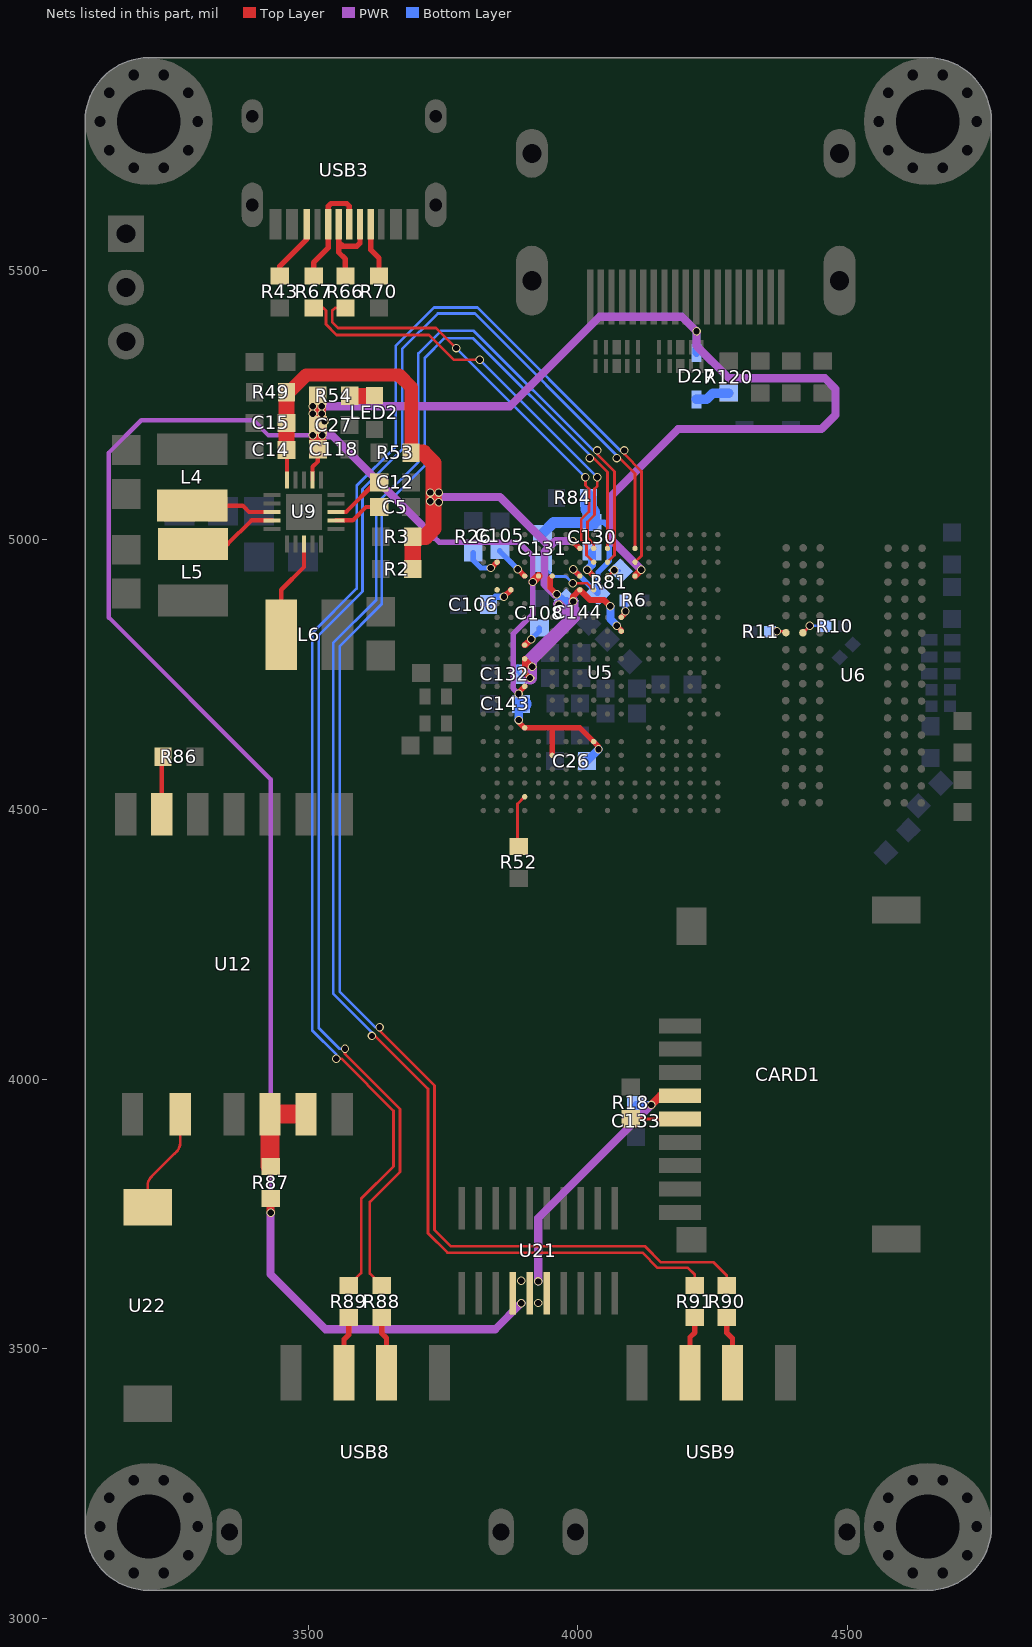
[diagram p0: the nets of this part, all layers, seen from the top]
# Altium PCB MISC105417.pcbdoc (part 2 of 5)
Units mil, origin at the board's own origin, x right, y up, seen from the top; angles counter-clockwise.
Board outline 1681.1 x 2842.52 mil, 4 copper layers (Top Layer, GND, PWR, Bottom Layer), stack 62.447 mil thick; 102 components, 152 nets, 737 pads, 611 vias.

## Footprints (in the part's own frame and the unit in brackets; to place one, negate y for a bottom-side part, rotate by r counter-clockwise, add the part's x,y. Pads: shape width x height; smd on the part's side, far side on the other; paste and mask are expansions set on the pad) (continued)
FBGA96 [mil]
  round 14 smd: A1(-128.47,241.36) A2(-96.97,241.37) A3(-65.47,241.38) A7(60.53,241.42) A8(92.03,241.43) A9(123.53,241.44) B1(-128.46,209.86) B2(-96.96,209.87) B3(-65.46,209.88) B7(60.54,209.92) B8(92.04,209.93) B9(123.54,209.94) C1(-128.46,178.36) C2(-96.96,178.37) C3(-65.46,178.38) C7(60.54,178.42) C8(92.04,178.43) C9(123.54,178.44) D1(-128.45,146.86) D2(-96.95,146.87) D3(-65.45,146.88) D7(60.55,146.92) D8(92.05,146.93) D9(123.55,146.94) E1(-128.44,115.36) E2(-96.94,115.37) E3(-65.44,115.38) E7(60.56,115.42) E8(92.06,115.43) E9(123.56,115.44) F1(-128.43,83.86) F2(-96.93,83.87) F3(-65.43,83.88) F7(60.57,83.92) F8(92.07,83.93) F9(123.57,83.94) G1(-128.42,52.36) G2(-96.92,52.37) G3(-65.42,52.38) G7(60.58,52.42) G8(92.08,52.43) G9(123.58,52.44) H1(-128.41,20.86) H2(-96.91,20.87) H3(-65.41,20.88) H7(60.59,20.92) H8(92.09,20.93) H9(123.59,20.94) J1(-128.4,-10.64) J2(-96.9,-10.63) J3(-65.4,-10.62) J7(60.6,-10.58) J8(92.1,-10.57) J9(123.6,-10.56) K1(-128.39,-42.14) K2(-96.89,-42.13) K3(-65.39,-42.12) K7(60.61,-42.08) K8(92.11,-42.07) K9(123.61,-42.06) L1(-128.38,-73.64) L2(-96.88,-73.63) L3(-65.38,-73.62) L7(60.62,-73.58) L8(92.12,-73.57) L9(123.62,-73.56) M1(-128.37,-105.14) M2(-96.87,-105.13) M3(-65.37,-105.12) M7(60.63,-105.08) M8(92.13,-105.07) M9(123.63,-105.06) N1(-128.36,-136.64) N2(-96.86,-136.63) N3(-65.36,-136.62) N7(60.64,-136.58) N8(92.14,-136.57) N9(123.64,-136.56) P1(-128.35,-168.14) P2(-96.85,-168.13) P3(-65.35,-168.12) P7(60.65,-168.08) P8(92.15,-168.07) P9(123.65,-168.06) R1(-128.34,-199.64) R2(-96.84,-199.63) R3(-65.34,-199.62) R7(60.66,-199.58) R8(92.16,-199.57) R9(123.66,-199.56) T1(-128.33,-231.14) T2(-96.83,-231.13) T3(-65.33,-231.12) T7(60.67,-231.08) T8(92.17,-231.07) T9(123.67,-231.06)
  silkscreen extent -180,-270 175,281
HDMI-SMD_HDMI-19PIN-043 [mm]
  rect 0.3x2.6 smd paste-100 mask+0.05: 1(4.5,3.38) 2(4,3.38) 3(3.5,3.38) 4(3,3.38) 5(2.5,3.38) 6(2,3.38) 7(1.5,3.38) 8(1,3.38) 9(0.5,3.38) 10(0,3.38) 11(-0.5,3.38) 12(-1,3.38) 13(-1.5,3.38) 14(-2,3.38) 15(-2.5,3.38) 16(-3,3.38) 17(-3.5,3.38) 18(-4,3.38) 19(-4.5,3.38)
  oval 1.5x2.3 hole 0.9 slot 1.7 at 90 deg paste+0 mask+0.05: 20(-7.25,-3.38) 20(7.25,-3.38)
  oval 1.5x3.3 hole 0.9 slot 2.7 at 90 deg paste+0 mask+0.05: 20(-7.25,2.62) 20(7.25,2.62)
  silkscreen extent -7.5,-7.88 7.5,4.92
hdr-th_3p-p2.54-v-m [mm]
  rect 1.7x1.7 hole 0.889 paste+0 mask+0.051: 1(-2.54,0)
  round 1.7 hole 0.889 paste+0 mask+0.051: 2(0,0) 3(2.54,0)
  silkscreen extent -4.02,-1.27 4.02,1.27
IND-SMD_L3.0-W3.0 [mm]
  rect 1.5x3.32 smd paste+0 mask+0.051: 1(1.328,0) 2(-1.328,0)
  silkscreen extent -1.52,-1.91 1.52,1.91
LED_0603 [mil]
  rect 31.5x31.5 smd paste+0 mask+2: 1(-33.5,-0.4) 2(29.5,-0.2)
  silkscreen extent -61,-30 53,30
M3_HOLE [mm]
  round 1 hole 0.5: 1(-2.3,0) 1(-1.861,-1.352) 1(-1.861,1.352) 1(-0.711,-2.187) 1(-0.711,2.187) 1(0.711,-2.187) 1(0.711,2.187) 1(1.861,-1.352) 1(1.861,1.352) 1(2.3,0)
  round 6 hole 3: 1(0,0)
OSC-SMD_4P-L2.0-W1.6-BL [mil]
  rect 30x20 smd: 1(-25,-20) 2(25,-20) 3(25,20) 4(-25,20)
R0402 [mm]
  rect 0.566x0.54 smd paste-100 mask+0.051: 1(-0.433,0) 2(0.433,0)
  silkscreen extent -0.94,-0.5 0.94,0.5
R0402-NSK_2 [mil]
  rect 19.68x22 smd paste+0 mask+2: 1(-18,0) 2(18,0)
R0603 [mil]
  rect 31.75x34.02 smd paste-3937.01 mask+2: 1(-29.66,0) 2(29.66,0)
  silkscreen extent -55,-26 55,26
SLP2510P8_L2.5-W1.0-P0.50-BL [mil]
  rect 7.9x26.8 smd paste+0 mask+2: 1(-39.4,-17.3) 2(-19.7,-17.3) 4(19.7,-17.3) 5(39.4,-17.3) 6(39.4,17.3) 7(19.7,17.3) 9(-19.7,17.3) 10(-39.4,17.3)
  rect 15.7x26.8 smd paste+0 mask+2: 3(0,-17.3) 8(0,17.3)
  silkscreen extent -57,-35 51,22
SOD-323_L1.8-W1.3-LS2.5-NSK [mil]
  rect 33.3x17.9 smd paste+0 mask+2: 1(-43.2,0) 2(43.2,0)
  silkscreen extent -18,-10 -6,7
TF-SMD_TF-015 [mil]
  rect 27.6x78.7 smd paste+0 mask+2: 1(90.7,200.6) 2(47.6,200.5) 3(4.4,200.6) 4(-38.8,200.6) 5(-82.1,200.6) 6(-125.3,200.6) 7(-168.5,200.6) 8(-211.7,200.6) 9(-255.2,200.6)
  rect 47.2x55 smd paste+0 mask+2: 10(-305.7,179.4)
  rect 50x90 smd paste+0 mask+2: 11(-304.3,-200.6) 12(305.7,-200.6)
  rect 70x55 smd paste+0 mask+2: 13(275.7,179.4)
  Board Outline Layer circle w0.1: c-192.8,-216.8 r19.7
  Board Outline Layer circle w0.1: c122.1,-216.7 r19.7
  Board Outline Layer region: -192.8,-236.5 -201.35,-234.55 -208.2,-229.08 -212.01,-221.18 -212.01,-212.42 -208.2,-204.52 -201.35,-199.05 -192.8,-197.1 -192.8,-197.1 -184.25,-199.05 -177.4,-204.52 -173.59,-212.42 -173.59,-221.18 -177.4,-229.08 -184.25,-234.55 -192.8,-236.5
  Board Outline Layer region: -192.8,-236.5 -196.64,-236.12 -200.34,-235 -203.74,-233.18 -206.73,-230.73 -209.18,-227.74 -211,-224.34 -212.12,-220.64 -212.5,-216.8 -212.12,-212.96 -211,-209.26 -209.18,-205.86 -206.73,-202.87 -203.74,-200.42 -200.34,-198.6 -196.64,-197.48 -192.8,-197.1 -188.96,-197.48 -185.26,-198.6 -181.86,-200.42 -178.87,-202.87 -176.42,-205.86 -174.6,-209.26 -173.48,-212.96 -173.1,-216.8 -173.48,-220.64 -174.6,-224.34 -176.42,-227.74 -178.87,-230.73 -181.86,-233.18 -185.26,-235 -188.96,-236.12
  Board Outline Layer region: 122.1,-236.4 113.55,-234.45 106.7,-228.98 102.89,-221.08 102.89,-212.32 106.7,-204.42 113.55,-198.95 122.1,-197 122.1,-197 130.65,-198.95 137.5,-204.42 141.31,-212.32 141.31,-221.08 137.5,-228.98 130.65,-234.45 122.1,-236.4
  Board Outline Layer region: 122.1,-236.4 118.26,-236.02 114.56,-234.9 111.16,-233.08 108.17,-230.63 105.72,-227.64 103.9,-224.24 102.78,-220.54 102.4,-216.7 102.78,-212.86 103.9,-209.16 105.72,-205.76 108.17,-202.77 111.16,-200.32 114.56,-198.5 118.26,-197.38 122.1,-197 125.94,-197.38 129.64,-198.5 133.04,-200.32 136.03,-202.77 138.48,-205.76 140.3,-209.16 141.42,-212.86 141.8,-216.7 141.42,-220.54 140.3,-224.24 138.48,-227.64 136.03,-230.63 133.04,-233.08 129.64,-234.9 125.94,-236.02
  Multi-Layer board cut-out: -192.8,-236.5 -201.35,-234.55 -208.2,-229.08 -212.01,-221.18 -212.01,-212.42 -208.2,-204.52 -201.35,-199.05 -192.8,-197.1 -192.8,-197.1 -184.25,-199.05 -177.4,-204.52 -173.59,-212.42 -173.59,-221.18 -177.4,-229.08 -184.25,-234.55 -192.8,-236.5
  Multi-Layer board cut-out: 122.1,-236.4 113.55,-234.45 106.7,-228.98 102.89,-221.08 102.89,-212.32 106.7,-204.42 113.55,-198.95 122.1,-197 122.1,-197 130.65,-198.95 137.5,-204.42 141.31,-212.32 141.31,-221.08 137.5,-228.98 130.65,-234.45 122.1,-236.4
  silkscreen extent -287,-376 295,165
USB-A-SMD_C42496 [mm]
  rect 1x2.6 smd paste-100 mask+0.05: 1(-3.5,3.75) 2(-1,3.75) 3(1,3.75) 4(3.5,3.75)
  oval 1.2x2.2 hole 0.8 slot 1.8 at 90 deg paste+0 mask+0.05: 5(-6.4,-3.75) 6(6.4,-3.75)
  silkscreen extent -7.15,-6.25 7.15,3.75
USB-C-SMD_TYPEC-304-BCP16-1 [mil]
  oval 39.4x82.7 hole 23.6 slot 66.9 at 90 deg paste+0 mask+1.97: 12(-170.1,64.3) 13(170.1,64.3)
  oval 39.4x63 hole 23.6 slot 47.2 at 90 deg paste+0 mask+1.97: 14(-170.1,-100.3) 15(170.1,-100.3)
  rect 21.7x57.1 smd paste-3937.01 mask+1.97: A1B12(-127,100.3) A4B9(-96.5,100.3) B1A12(127,100.3) B4A9(96.5,100.3)
  rect 11.8x57.1 smd paste-3937.01 mask+1.97: A5(-49.2,100.3) A6(-9.8,100.3) A7(9.8,100.3) A8(49.2,100.3) B5(68.9,100.3) B6(29.5,100.3) B7(-29.5,100.3) B8(-68.9,100.3)
  Board Outline Layer circle w0.1: c-113.8,43.4 r12.8
  Board Outline Layer circle w0.1: c113.8,43.4 r12.8
  Board Outline Layer region: -126.6,43.4 -125.33,48.95 -121.78,53.41 -116.65,55.88 -110.95,55.88 -105.82,53.41 -102.27,48.95 -101,43.4 -101,43.4 -102.27,37.85 -105.82,33.39 -110.95,30.92 -116.65,30.92 -121.78,33.39 -125.33,37.85 -126.6,43.4
  Board Outline Layer region: -126.6,43.4 -126.23,46.46 -125.13,49.35 -123.38,51.89 -121.07,53.93 -118.34,55.37 -115.34,56.11 -112.26,56.11 -109.26,55.37 -106.53,53.93 -104.22,51.89 -102.47,49.35 -101.37,46.46 -101,43.4 -101.37,40.34 -102.47,37.45 -104.22,34.91 -106.53,32.87 -109.26,31.43 -112.26,30.69 -115.34,30.69 -118.34,31.43 -121.07,32.87 -123.38,34.91 -125.13,37.45 -126.23,40.34
  Board Outline Layer region: 101,43.4 102.27,48.95 105.82,53.41 110.95,55.88 116.65,55.88 121.78,53.41 125.33,48.95 126.6,43.4 126.6,43.4 125.33,37.85 121.78,33.39 116.65,30.92 110.95,30.92 105.82,33.39 102.27,37.85 101,43.4
  Board Outline Layer region: 101,43.4 101.37,46.46 102.47,49.35 104.22,51.89 106.53,53.93 109.26,55.37 112.26,56.11 115.34,56.11 118.34,55.37 121.07,53.93 123.38,51.89 125.13,49.35 126.23,46.46 126.6,43.4 126.23,40.34 125.13,37.45 123.38,34.91 121.07,32.87 118.34,31.43 115.34,30.69 112.26,30.69 109.26,31.43 106.53,32.87 104.22,34.91 102.47,37.45 101.37,40.34
  Multi-Layer board cut-out: -126.6,43.4 -125.33,48.95 -121.78,53.41 -116.65,55.88 -110.95,55.88 -105.82,53.41 -102.27,48.95 -101,43.4 -101,43.4 -102.27,37.85 -105.82,33.39 -110.95,30.92 -116.65,30.92 -121.78,33.39 -125.33,37.85 -126.6,43.4
  Multi-Layer board cut-out: 101,43.4 102.27,48.95 105.82,53.41 110.95,55.88 116.65,55.88 121.78,53.41 125.33,48.95 126.6,43.4 126.6,43.4 125.33,37.85 121.78,33.39 116.65,30.92 110.95,30.92 105.82,33.39 102.27,37.85 101,43.4
  silkscreen extent -173,-203 173,16
WIFI模块 [mm]
  rect 2x1 smd: 1(1.947,-1.15) 2(1.947,-2.85) 3(1.947,-4.55) 4(1.947,-6.25) 5(1.947,-7.95) 6(1.947,-9.65) 7(1.947,-11.35) 8(16.08,-11.03) 9(16.08,-8.78) 10(16.08,-6.25) 11(16.08,-4.55) 12(16.08,-2.85) 13(16.08,-1.15)
  silkscreen extent -0.3,-12.5 16.08,0
WQFN-20_L3.0-W3.0-P0.40-BL-EP [mil]
  rect 7.9x31.5 smd paste+0 mask+2: 1(-31.5,-59.1) 2(-15.8,-59.1) 3(0,-59.1) 4(15.7,-59.1) 5(31.5,-59.1) 11(31.5,59.1) 12(15.7,59.1) 13(0,59.1) 14(-15.8,59.1) 15(-31.5,59.1)
  rect 31.5x7.9 smd paste+0 mask+2: 6(59.1,-31.5) 7(59.1,-15.7) 8(59.1,0) 9(59.1,15.7) 10(59.1,31.5) 16(-59.1,31.5) 17(-59.1,15.8) 18(-59.1,0) 19(-59.1,-15.7) 20(-59.1,-31.5)
  rect 66.9x66.9 smd paste+0 mask+2: 21(0,0)
  silkscreen extent -61,-83 61,61

## Via types
v1: diameter 15.7, hole 11.8, Top Layer to Bottom Layer, 611 vias

## Nets (pads, with @x,y where several pads share a name; then routed paths per layer and width w, separated by ;. In a path a pad name is that pad's centre, name@x,y a point inside that pad or via, vN(x,y) a via of type N, cw(c..) or ccw(c..) an arc to the next point about the centre after c; other vN are vias at no path point)
1V8: C14.2 C15.2 C132.1 C144.2 R2.1 R3.1 R49.2 R53.1 U5.D11 U5.D12 U5.F18 U5.H17 U5.H20 U5.L14 U9.15 | length 1780.8
  Top Layer w8: C14.2@3459.53,5167 3460.5,5166.03 U9.15@3460.5,5111.1
  Top Layer w10: v1(3911.2,4743.94) 3911.2,4744.05 U5.D11@3901.25,4754 U5.D12@3901.25,4779.59 3915.2,4765.64 v1(3915.2,4764.94) ; U5.F18@3952.43,4933.13 3949,4929.7 3949,4910.97 v1(3960.65,4899.32) ; v1@3990,4997.92 U5.H20@4003.61,4984.31 ; v1(4072.2,4840.94) 4080.39,4832.77 U5.L14@4080.39,4830.77
  Top Layer w11: v1(3991.2,4885.94) 3991.2,4895.13 U5.H17@4003.61,4907.54 4022.21,4888.94 4048.2,4888.94 v1(4060.2,4876.94)
  Top Layer w25: R49.2@3459.66,5274 3464,5274 3496,5306 3668,5306 3690.66,5283.34 R53.1@3690.66,5162
  Top Layer w30: C14.2@3459.53,5167 3459.66,5167.13 R49.2@3459.66,5274 ; R53.1@3690.66,5162 3713,5162 3732,5143 3732,5021 3717,5006 R3.1@3693.66,5006 R2.1@3693.66,4946
  PWR w15: 3728,5080 3855.15,5080 3947.6,4987.54 ; v1(3960.65,4899.32) 3956.68,4899.32 3938,4918 3938,4977.94 3947.6,4987.54 ; v1(3990,4998) 3958.06,4998 3947.6,4987.54
  PWR w20: v1(3964.2,4879.94) 3975.83,4868.32 3991.2,4868.32 v1(3991.2,4885.94)
  PWR w25: v1(3911.2,4743.94) 3911.2,4776.94 3991.2,4856.94 3991.2,4868.32
  Bottom Layer w5: C132.1@3888.2,4766.94 3888.2,4754.79 C132.1@3892.08,4750.91 3892.08,4744.82 C132.1@3889.2,4741.94 ; C144.2@3978.64,4886.79 3979.49,4885.94 v1(3991.2,4885.94)
  Bottom Layer w10: v1(3964.2,4879.94) 3971.79,4879.94 C144.2@3978.64,4886.79
  Bottom Layer w15: v1(3960.65,4899.32) 3973.18,4886.79 C144.2@3978.64,4886.79 ; v1(4060.2,4876.94) 4060.2,4852.94 v1(4072.2,4840.94)
  other v1: 3742,5070 3726,5072 3726,5088 3742,5088
3V3: C26.2 C27.2 C118.2 C133.2 C143.2 CARD1.4 D27.2 R54.2 R87.1 U5.D7 U5.D10 U5.E18 U5.F5 U5.J6 U5.M18 U9.12 U21.4 U21.5 U21.6 | length 6238
  Top Layer w8: U9.12@3507.7,5111.1 3507.7,5135.7 3517.63,5145.63 C118.2@3517.63,5168.29
  Top Layer w10: v1(3889.91,4714.61) 3889.91,4717.07 U5.D10@3901.25,4728.41 ; v1(3890.2,4665.94) 3890.2,4662.69 U5.D7@3901.25,4651.64 3952.43,4651.64 ; U5.F5@3952.43,4600.46 3952.43,4651.64 ; v1(4038.2,4611.94) 4038.2,4617.05 U5.J6@4029.2,4626.05 4003.61,4651.64 3952.43,4651.64
  Top Layer w12: U5.M18@4105.98,4933.13 4117.2,4944.35 v1(4117.2,4944.94)
  Top Layer w15: v1(3430,3752) R87.1@3430,3778.34 ; v1(3916,4922) 3916,4922.29 U5.E18@3926.84,4933.13 ; v1(4136,3952) 4153.2,3969.2 CARD1.4@4189.4,3969.2
  Top Layer w30: R54.2@3517.5,5267.29 C27.2@3517.47,5213 3517.5,5168.42 C118.2@3517.63,5168.29
  PWR w8: v1(3430,3752) 3430,4556 3130,4856 3130,5162 3190,5222 3398.1,5222 3426.1,5194 v1(3508,5194)
  PWR w10: 3732.41,5006 3742.41,4996 3890,4996 3916,4970 v1(3916,4922) 3916,4862 3880,4826 3880,4724.52 v1(3889.91,4714.61)
  PWR w15: v1(3430,3752) 3430,3638 3532,3536 3846.63,3536 v1(3895,3584.37) ; v1(3508,5194) v1(3526.04,5194) 3544.41,5194 3732.41,5006 ; v1(3525.18,5248) 3874,5248 4040,5414 4193.19,5414 v1(4220,5387.19) 4220,5360 4280,5300 4458,5300 4478,5280 4478,5232 4452,5206 4186,5206 4063,5083 4063,4999.15 v1(4117.2,4944.94) ; v1(3926.44,3624.66) 3926.44,3742.44 v1(4136,3952)
  Bottom Layer w5: v1(3889.91,4714.61) 3889.91,4700.35 C143.2@3894.35,4695.91
  Bottom Layer w15: v1(3890.2,4665.94) 3890.2,4691.76 C143.2@3894.35,4695.91 ; C26.2@4016.73,4589.94 4038.2,4611.41 v1(4038.2,4611.94) ; C133.2@4108,3951.53 4108.47,3952 v1(4136,3952) ; D27.2@4220,5347.2 v1(4220,5387.19)
  Bottom Layer w30: C143.2@3894.35,4695.91 C143.2@3899.24,4695.91
  other v1: 3926.44,3584.66 3895,3626 3530,5220 3508,5234 3524.57,5234 3508,5248
$1N1032: R6.1 U5.L15 | length 35.5
  Top Layer w10: U5.L15@4080.39,4856.36 4088.2,4864.17 v1(4088.2,4867.94)
  Bottom Layer w10: R6.1@4086.52,4887.91 4086.52,4869.62 v1(4088.2,4867.94)
$1N2048: R10.2 U6.L8 | length 47.8
  Top Layer w5: U6.L8@4417.34,4827.89 4430.2,4840.76 v1(4430.2,4840.94)
  Bottom Layer w5: v1(4430.2,4840.94) 4458.16,4840.94 R10.2@4459.16,4839.94
$1N2049: R11.2 U6.L9 | length 17.9
  Top Layer w5: v1(4369.2,4830.94) 4382.89,4830.94 U6.L9@4385.84,4827.99
$2N1493: LED2.2 R54.1 | length 45.7
  Top Layer w30: R54.1@3576.82,5267.29 3621.86,5267.29 LED2.2@3622.36,5267.79
$2N1502: C12.2 U9.8 | length 103.2
  Top Layer w8: U9.8@3551.1,5052 3570,5052 3625,5107 C12.2@3631.47,5107
$2N1513: C5.2 U9.7 | length 90.6
  Top Layer w8: U9.7@3551.1,5036.3 3582.3,5036.3 3607,5061 C5.2@3631.47,5061
$2N1522: L6.1 U9.3 | length 186.4
  Top Layer w8: L6.1@3449.72,4824 3449.72,4907.72 3492,4950 U9.3@3492,4992.9
$2N1523: L5.1 U9.19 | length 165.1
  Top Layer w8: L5.1@3286,4992.28 3350.28,4992.28 3394.3,5036.3 U9.19@3432.9,5036.3
$2N1524: L4.1 U9.18 | length 152.8
  Top Layer w8: L4.1@3285,5063.72 3378.28,5063.72 3390,5052 U9.18@3432.9,5052
$3N1343: C130.2 U5.J18 | length 53.1
  Top Layer w10: v1(4017.2,4944.94) 4017.39,4944.94 U5.J18@4029.2,4933.13
  Bottom Layer w15: v1(4017.2,4944.94) 4026.2,4953.94 C130.2@4026.2,4977.38
$3N1344: C131.2 U5.J17 | length 117.5
  Top Layer w5: v1(3990.2,4919.94) 4016.8,4919.94 U5.J17@4029.2,4907.54
  Bottom Layer w5: C131.2@3934,4956.44 3934,4952.93 3954.66,4932.27 3977.88,4932.27 v1(3990.2,4919.94)
$3N1345: R81.2 U5.K18 | length 27.3
  Top Layer w5: U5.K18@4054.8,4933.13 4056.39,4933.13 v1(4067.2,4943.94)
  Bottom Layer w5: v1(4067.2,4943.94) 4076.15,4943.94 R81.2@4077.18,4942.91
$3N1352: C105.2 U5.D18 | length 66.5
  Top Layer w10: v1(3888.2,4945.94) 3888.44,4945.94 U5.D18@3901.25,4933.13
  Bottom Layer w10: C105.2@3855.2,4980.38 3855.2,4978.94 v1(3888.2,4945.94)
$3N1353: C106.2 U5.C17 | length 54.4
  Top Layer w10: v1(3862.8,4894.72) U5.C17@3875.62,4907.54
  Bottom Layer w12: C106.2@3833.76,4879.94 3833.76,4881.76 3846.72,4894.72 v1(3862.8,4894.72)
$3N1362: C108.1 U5.D13 | length 43.2
  Top Layer w12: U5.D13@3901.25,4805.18 3902.44,4805.18 v1(3913.2,4815.94)
  Bottom Layer w10: v1(3913.2,4815.94) 3928.52,4831.26 C108.1@3928.52,4836.35
$3N1420: R43.1 USB3.B5 | length 116.5
  Top Layer w10: R43.1@3447.03,5489.74 3447.03,5508.03 3497.3,5558.3 USB3.B5@3497.3,5585.45
$3N1449: R70.2 USB3.A5 | length 102.2
  Top Layer w10: USB3.A5@3615.4,5585.45 3615.4,5538.6 3631.03,5522.97 R70.2@3631.03,5489.74
$3N15581: D27.1 R120.1 | length 64.8
  Bottom Layer w18: D27.1@4220,5260.8 4238.8,5260.8 4250.34,5272.34 R120.1@4280,5272.34
$4N793: R52.1 U5.D2 | length 98.3
  Top Layer w5: R52.1@3890,4431.66 3888,4433.66 3888,4510.44 U5.D2@3901.25,4523.69
$4N2263: CARD1.5 R18.2 | length 91.6
  Top Layer w5: R18.2@4098,3926.34 4098.44,3925.9 CARD1.5@4189.4,3925.9
$4N8011: R86.1 U12.6 | length 107.6
  Top Layer w8: U12.6@3228.08,4491.33 3228.08,4595.74 R86.1@3230.34,4598
$4N8060: R87.2 U12.11 U12.12 | length 164.6
  Top Layer w35: R87.2@3430,3837.66 3428.87,3838.79 U12.11@3428.87,3934.91 U12.12@3495.8,3934.91
$4N8418: U12.9 U22.1 | length 195.8
  Top Layer w5: U22.1@3202,3762.28 3202,3802 ; 3202,3802.81 cw(c3224.42,3802.74) 3209.27,3819.27 ; 3209,3819 3252,3862 ccw(c3237.16,3882.35) 3262.33,3881.54 ; 3262.33,3881 U12.9@3262.33,3934.91
AGND: C130.1 C131.1 R81.1 R84.2 U5.H18 | length 398.2
  Top Layer w10: v1(3991.2,4945.94) 3991.2,4945.54 U5.H18@4003.61,4933.13
  Bottom Layer w10: v1(3991.2,4945.94) 4036.18,4900.97 R81.1@4037.23,4900.97 4037.23,4939.97 4058.2,4960.94 4058.2,5022.94 4048.64,5032.5 C130.1@4026.2,5032.5
  Bottom Layer w20: C131.1@3934,5011.56 3954.94,5032.5 C130.1@4026.2,5032.5
  Bottom Layer w30: R84.2@4019.86,5077.94 4019.86,5057.28 4026.2,5050.94 C130.1@4026.2,5032.5
D0+: R67.2 USB3.A6 USB3.B6 | length 217.3
  Top Layer w10: R67.2@3509.7,5489.74 3509.7,5514.7 3536.7,5541.7 USB3.B6@3536.7,5585.45 3536.7,5618.7 3542,5624 3571,5624 3576,5619 USB3.A6@3576,5585.45
D0-: R66.2 USB3.A7 USB3.B7 | length 180.4
  Top Layer w10: USB3.A7@3556.4,5585.45 3556.4,5552.6 ; R66.2@3568.75,5489.74 3568.75,5521.25 3556.4,5533.6 3556.4,5552.6 ; USB3.B7@3595.7,5585.45 3595.7,5550.7 3590,5545 3564,5545 3556.4,5552.6
D0C+: R67.1 U5.J20 | length 815.3
  Top Layer w5: R67.1@3509.7,5430.42 3527.58,5430.42 3532.71,5425.29 3532.71,5400.14 3552.51,5380.34 3723.66,5380.34 3770,5334 v1(3818,5334) ; U5.J20@4029.2,4984.31 4029.2,4992.8 4017.7,5004.3 4017.7,5033.7 4030.69,5046.69 4030.69,5094.82 4036,5100.13 v1(4036,5116)
  Bottom Layer w5: v1(3818,5334) v1(4036,5116)
D0C-: R66.1 U5.J19 | length 812.5
  Top Layer w5: R66.1@3568.75,5430.42 3549.44,5430.42 3544.16,5425.14 3544.16,5404.12 3555.1,5393.18 3736.82,5393.18 v1(3774,5356) ; v1(4014,5116) 4014,5101.24 4020.47,5094.77 4020.47,5052.47 4006,5038 4006,5000 4016,4990 4016,4971.92 U5.J19@4029.2,4958.72
  Bottom Layer w5: v1(3774,5356) v1(4014,5116)
D1+: R88.2 USB8.3 | length 105.9
  Top Layer w10: R88.2@3636.03,3557.66 3636.03,3528.66 3644.94,3519.74 USB8.3@3644.94,3455.43
D1-: R89.2 USB8.2 | length 105.9
  Top Layer w10: USB8.2@3566.2,3455.43 3566.2,3517.2 3575.03,3526.03 R89.2@3575.03,3557.66
D1C+: R88.1 U5.M20 | length 2625.9
  Top Layer w5: v1(3568,4056) 3568,4046.39 3670,3944.39 3670,3828 3614,3772 3614,3639.01 R88.1@3636.03,3616.98 ; v1(4072,5152) 4076.87,5152 4105.98,5122.89 U5.M20@4105.98,4984.31
  Bottom Layer w5: v1(3568,4056) 3558.26,4056 3519.04,4095.22 3519.04,4823.04 3600.29,4904.29 3600.29,5094.35 3674,5168.06 3674,5354 3740.24,5420.24 3808.84,5420.24 4072,5157.07 v1(4072,5152)
D1C-: R89.1 U5.M19 | length 2698.1
  Top Layer w5: v1(3552,4038) 3561.07,4038 3658,3941.07 3658,3838 3598,3778 3598,3639.94 R89.1@3575.03,3616.98 ; v1(4086,5166) 4086,5159.23 4118,5127.23 4118,4970.74 U5.M19@4105.98,4958.72
  Bottom Layer w5: v1(3552,4038) 3552,4045.4 3507.24,4090.15 3507.24,4827.24 3589.71,4909.71 3589.71,5100.58 3662.3,5173.18 3662.3,5360.3 3733.22,5431.22 3813.34,5431.22 4078.56,5166 v1(4086,5166)
D3+: R90.2 USB9.3 | length 106.6
  Top Layer w10: R90.2@4276.02,3557.66 4276.02,3529.62 4286.68,3518.96 USB9.3@4286.68,3455.43
D3-: R91.2 USB9.2 | length 106
  Top Layer w10: USB9.2@4207.94,3455.43 4207.94,3521.12 4216.97,3530.15 R91.2@4216.97,3557.66
D3C+: R90.1 U5.K20 | length 2957.9
  Top Layer w5: v1(3632,4096) 3632,4089.78 3734,3987.78 3734,3720 3764,3690 4124,3690 4154,3660 4252,3660 4276.02,3635.98 R90.1@4276.02,3616.98 ; v1(4022,5152) 4028.49,5152 4054.8,5125.69 U5.K20@4054.8,4984.31
  Bottom Layer w5: v1(3632,4096) 3624.56,4096 3558,4162.56 3558,4802.79 3636,4880.79 3636,5057.76 3716,5137.76 3716,5338 3752,5374 3805.82,5374 4022,5157.82 v1(4022,5152)
D3C-: R91.1 U5.K19 | length 2988.1
  Top Layer w5: v1(3618,4080) 3623.95,4080 3722,3981.95 3722,3714 3758,3678 4120,3678 4148,3650 4204,3650 4216.97,3637.03 R91.1@4216.97,3616.98 ; v1(4036,5166) 4036,5158.93 4068,5126.93 4068,4971.92 U5.K19@4054.8,4958.72
  Bottom Layer w5: v1(3618,4080) 3618,4086.63 3546,4158.63 3546,4808.49 3625.65,4888.14 3625.65,5066.63 3704,5144.98 3704,5346 3746,5388 3806.83,5388 4028.83,5166 v1(4036,5166)
EPHY_RTX: R26.1 U5.B19 | length 68.6
  Top Layer w10: v1(3838,4948) 3839.35,4948 U5.B19@3850.07,4958.72
  Bottom Layer w10: R26.1@3806,4976.34 3806,4962 3820,4948 v1(3838,4948)
FEL: U5.B17